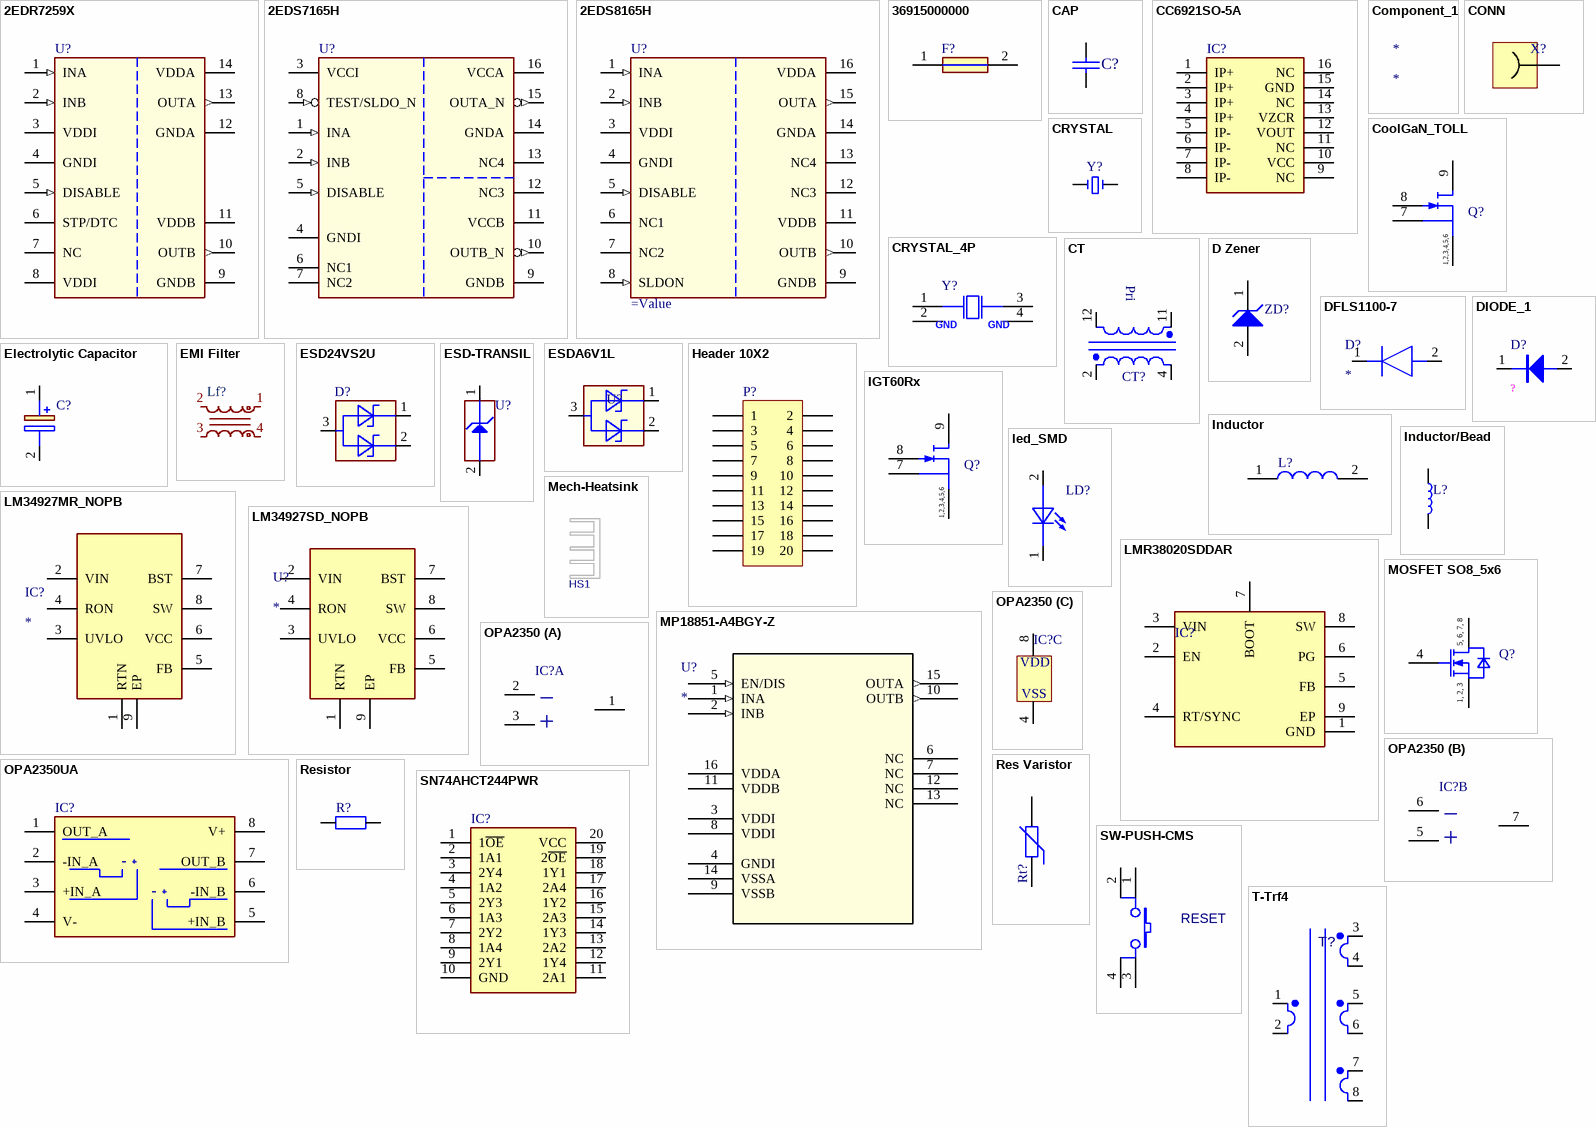
[diagram p0: symbols 2EDR7259X to T-Trf4]
# Altium schematic symbol library MISC82254-2.SchLib: 50 symbols
Pins are listed as number, name and electrical type; pins without a type are passive.


## 2EDR7259X
designator U?
Dual-Channel Isolated Gate Driver
footprint SOIC127P1030X265-16_14N-V (SOIC,1.27mm,pitch;14 pin,7.50mm W X 10.30mm L X 2.65mm H body)
pins: 1 INA (in) "Input signal channel A", 2 INB (in) "Input signal channel B", 3 VDDI (power) "Input-side supply voltage", 4 GNDI (power) "Ground primary-side", 5 DISABLE (in) "Disable input channel A and B", 6 STP/DTC "Shoot-through Protection and Dead-Time Control", 7 NC "No internal connection", 8 VDDI (power) "Input-side supply voltage", 9 GNDB (power) "Ground secondary-side channel B", 10 OUTB (out) "Output secondary-side channel B", 11 VDDB (power) "Supply secondary-side channel B", 12 GNDA (power) "Ground secondary-side channel A", 13 OUTA (out) "Output secondary-side channel A", 14 VDDA (power) "Supply voltage for output channel A"

## 2EDS7165H
designator U?
EiceDRIVER, Two Channel Isolated ISO Driver
footprint SOIC127P1030X265-16N-V (SOIC,1.27mm pitch;16 pin,7.50mm W X 10.30mm L X 2.65mm H body)
pins: 1 INA (in) "Input signal channel A", 2 INB (in) "Input signal channel B", 3 VCCI (power) "Positive supply voltage on input side", 4 GNDI (power) "Ground on input side", 5 DISABLE (in) "Input signal channel A and B", 6 NC1 "Not connected", 7 NC2 "Not connected", 8 TEST/SLDO_N (in) "Switch LDO on, low active or keep it floating / not connected", 9 GNDB (power) "Ground on output side for channel B", 10 OUTB_N (out) "Output driver for channel B", 11 VCCB (power) "Positive supply voltage on output side for channel B", 12 NC3 "Not connected", 13 NC4 "Not connected", 14 GNDA (power) "Ground on output side for channel A", 15 OUTA_N (out) "Output driver for channel A", 16 VCCA (power) "Positive supply voltage on output side for channel A"

## 2EDS8165H
designator U?
Dual-Channel, Functional and Reinforced Isolated MOSFET Gate-Driver
footprint PG-DSO-16 (SOIC,1.27mm pitch;16 pin,7.50mm W X 10.30mm L X 2.65mm H body)
pins: 1 INA (in) "Digital CMOS / TTL logic signal input for channel A with internal pull-down resistor to GNDI", 2 INB (in) "Digital CMOS / TTL logic signal input for channel B with internal pull-down resistor to GNDI", 3 VDDI (power) "Supply voltage (input side) 3.3 V (Internal SLDO available)", 4 GNDI (power) "Ground input side", 5 DISABLE (in) "Digital CMOS / TTL logic input for both channels A and B; logic input high disables both output channels", 6 NC1 "Not connected; keep pin floating", 7 NC2 "Not connected; keep pin floating", 8 SLDON (in) "Default 3.3 V supply selected, if N.C. or connected to VDDI", 9 GNDB (power) "Ground for output channel B", 10 OUTB (out) "Output gate driver for channel B", 11 VDDB (power) "Supply voltage for output channel B", 12 NC3 "Not present; not connected; for channel-to-channel isolation", 13 NC4 "Not connected; for channel-to-channel isolation", 14 GNDA (power) "Ground for output channel A", 15 OUTA (out) "Output gate driver for channel A", 16 VDDA (power) "Supply voltage for output channel A"

## 36915000000
designator F?
Fuse
footprint 36915000000
pins: 1, 2

## CAP
designator C?
footprint 0402C
footprint 0603C
footprint 0805C
footprint 1206C
footprint 1210C (capacitor 1210 reflow soldering)
footprint 2220
footprint CAPE
pins: 1, 2

## CC6921SO-5A
designator IC?
Integrated Circuit
footprint SOIC-16-300mil
pins: 1 IP+, 2 IP+, 3 IP+, 4 IP+, 5 IP-, 6 IP-, 7 IP-, 8 IP-, 9 NC, 10 VCC, 11 NC, 12 VOUT, 13 VZCR, 14 NC, 15 GND, 16 NC

## Component_1
designator *

## CONN
designator X?
footprint CONN_T44008
footprint Con_74650073R
pins: 1

## CoolGaN_TOLL
designator Q?
Field-Effect Transistor (FET), N-Channel, Enhancement, Pin 1-6 Source, Pin 7 kelvin Source, Pin 8 Gate, Pin 9 Drain, 9pins
footprint INF-PG-HSOF-8 (Transistor; 9 pin, 10.375 mm L X 9.90 mm W X 2.40 mm H body)
pins: 1 S1 "Source", 2 S2 "Source", 3 S3 "Source", 4 S4 "Source", 5 S5 "Source", 6 S6 "Source", 7 SK "Kelvin Source", 8 G "Gate", 9 D "DRAIN"

## CRYSTAL
designator Y?
Crystal
footprint XTAL-SMD-NX3215SA-32.768K-STD-MUS-2 (Crystal; 3.2mm W X 1.5mm L X 0.9mm H body)
pins: 1, 2

## CRYSTAL_4P
designator Y?
SMD Crystal Unit for Automotive Application, 12.000MHz; Version Number: V01
footprint XTAL-SMD-NX3225SA
pins: 1, 2 (power) "Ground", 3, 4 (power) "Ground"

## CT
designator CT?
Current transformer
pins: 2, 4, 11, 12

## D Zener
designator ZD?
Zener Diode
simulation model ZENER (Diode)
signal-integrity model D Zener
footprint SOD-323
pins: 1 A, 2 K

## DFLS1100-7
designator D?
Diode
footprint POWERDI123_1
pins: 1 K, 2 A

## DIODE_1
designator D?, comment ?
footprint SOD-323
footprint POWERDI123_1
footprint SMA
footprint SMA_L4.3-W2.6-LS5.2-RD
pins: 1 K, 2 A

## Electrolytic Capacitor
designator C?
Capacitor Polarised
footprint CAPPRD1000W190D3575H3200
pins: 1 +, 2 -

## EMI Filter
designator Lf?
pins: 1, 2, 3, 4

## ESD24VS2U
designator D?
Silicon TVS Diode, VRWM 24V
footprint SOT95P240X110-3N-1-V
pins: 1 CATHODE1 "Cathode", 2 CATHODE2 "Cathode", 3 ANODE "Anode"

## ESD-TRANSIL
designator U?
ESD protection 6V1
footprint ESD_ST0201
pins: 1 IO1, 2 GND

## ESDA6V1L
designator U?
No Description Available
footprint SOT_DA6V1L_STM
pins: 1 CATHODE1 "Cathode", 2 CATHODE2 "Cathode", 3 ANODE "Anode"

## Header 10X2
designator P?
Header, 10-Pin, Dual row
footprint HDR2X10 (Connector; Header; 10x2 Position)
pins: 1, 2, 3, 4, 5, 6, 7, 8, 9, 10, 11, 12, 13, 14, 15, 16, 17, 18, 19, 20

## IGT60Rx
designator Q?
Field-Effect Transistor (FET), N-Channel, Enhancement, Pin 1-6 Source, Pin 7 kelvin Source, Pin 8 Gate, Pin 9 Drain, 9pins
footprint INF-PG-HSOF-8 (Transistor; 9 pin, 10.375 mm L X 9.90 mm W X 2.40 mm H body)
pins: 1 S1 "Source", 2 S2 "Source", 3 S3 "Source", 4 S4 "Source", 5 S5 "Source", 6 S6 "Source", 7 SK "Kelvin Source", 8 G "Gate", 9 D "DRAIN"

## Inductor
designator L?
Inductor
pins: 1, 2

## Inductor/Bead
designator L?
footprint 0603R
pins: 1, 2
2 alternate drawings of the same symbol

## led_SMD
designator LD?
Version Number: V01
footprint LED0603-RD
pins: 1 Cathode, 2 Anode

## LM34927MR_NOPB
designator IC?
Integrated Circuit
footprint SOIC127P600X170-9N
pins: 1 RTN, 2 VIN, 3 UVLO, 4 RON, 5 FB, 6 VCC, 7 BST, 8 SW, 9 EP

## LM34927SD_NOPB
designator U?
Integrated Circuit
footprint WSON8
pins: 1 RTN, 2 VIN, 3 UVLO, 4 RON, 5 FB, 6 VCC, 7 BST, 8 SW, 9 EP

## LMR38020SDDAR
designator IC?
Integrated Circuit
footprint SO-8-PowerPad
pins: 1 GND, 2 EN, 3 VIN, 4 RT/SYNC, 5 FB, 6 PG, 7 BOOT, 8 SW, 9 EP

## Mech-Heatsink
designator HS1
Heatsink kit with Heatsink, Silpad and Clip
footprint Heatsink 15x15
footprint Heatsink 16x36x12(h) (4mm elevated)
footprint Heatsink 39x27.5mm (Manufactured from CTS BDN18-6CB/A01)
footprint Heatsink 46x28.5mm (Manufactured from CTS BDN18-6CB/A01)
footprint Heatsink 55x28.5 (1mm copper sheet)
footprint Heatsink C1613-001-04

## MOSFET SO8_5x6
designator Q?
MOSFET SO8 5x6
footprint IFX-PG-TDSON-8-36-V (PG-TDSON-8-36, SMD, 1.27 mm pitch, 8 pin, 5.90 mm L X 5.15 mm W X 1.00 mm H body)
pins: 1 SOURCE, 2 SOURCE, 3 SOURCE, 4 GATE, 5 DRAIN, 6 DRAIN, 7 DRAIN, 8 DRAIN

## MP18851-A4BGY-Z
designator U?
No Description Available
footprint SOIC-16WB_MP18851_MNP
pins: 1 INA (in), 2 INB (in), 3 VDDI (power), 4 GNDI (power), 5 EN/DIS (in), 6 NC, 7 NC, 8 VDDI (power), 9 VSSB (power), 10 OUTB (out), 11 VDDB (power), 12 NC, 13 NC, 14 VSSA (power), 15 OUTA (out), 16 VDDA (power)

## OPA2350
designator IC?
Dual op amp
footprint SOIC127P600X175-8N
part A pins: 1, 2, 3
part B pins: 5, 6, 7
part C pins: 4, 8

## OPA2350UA
designator IC?
Integrated Circuit
footprint SOIC127P600X175-8N
pins: 1 OUT_A, 2 -IN_A, 3 +IN_A, 4 V-, 5 +IN_B, 6 -IN_B, 7 OUT_B, 8 V+

## Res Varistor
designator Rt?
Thermistor
footprint RES-TH_Vol
footprint RV1-7.5MM
footprint R0603T
footprint 0603R
pins: 1, 2

## Resistor
designator R?
Resistor
signal-integrity model Res
simulation model RESISTOR
footprint 0402R
footprint 0603R
footprint 0805R
footprint 1206R
footprint 1210R
footprint 2220
pins: 1, 2

## SN74AHCT244PWR
designator IC?
Integrated Circuit
footprint TSSOP-20_L6.5-W4.4-P0.65-LS6.4-BL
pins: 1 1~{OE}, 2 1A1, 3 2Y4, 4 1A2, 5 2Y3, 6 1A3, 7 2Y2, 8 1A4, 9 2Y1, 10 GND, 11 2A1, 12 1Y4, 13 2A2, 14 1Y3, 15 2A3, 16 1Y2, 17 2A4, 18 1Y1, 19 2~{OE}, 20 VCC

## SW-PUSH-CMS
designator RESET
Non-Open Push-Button 0.1A 24V BLACK
footprint PTS647SM38SMTR2LFS
pins: 1, 2, 3, 4

## T-Trf4
designator T?
MAG-1238 13V to 12V
footprint Trans_isoBuck_MOS - EE25/20
pins: 1, 2, 3, 4, 5, 6, 7, 8

## T-Trf6
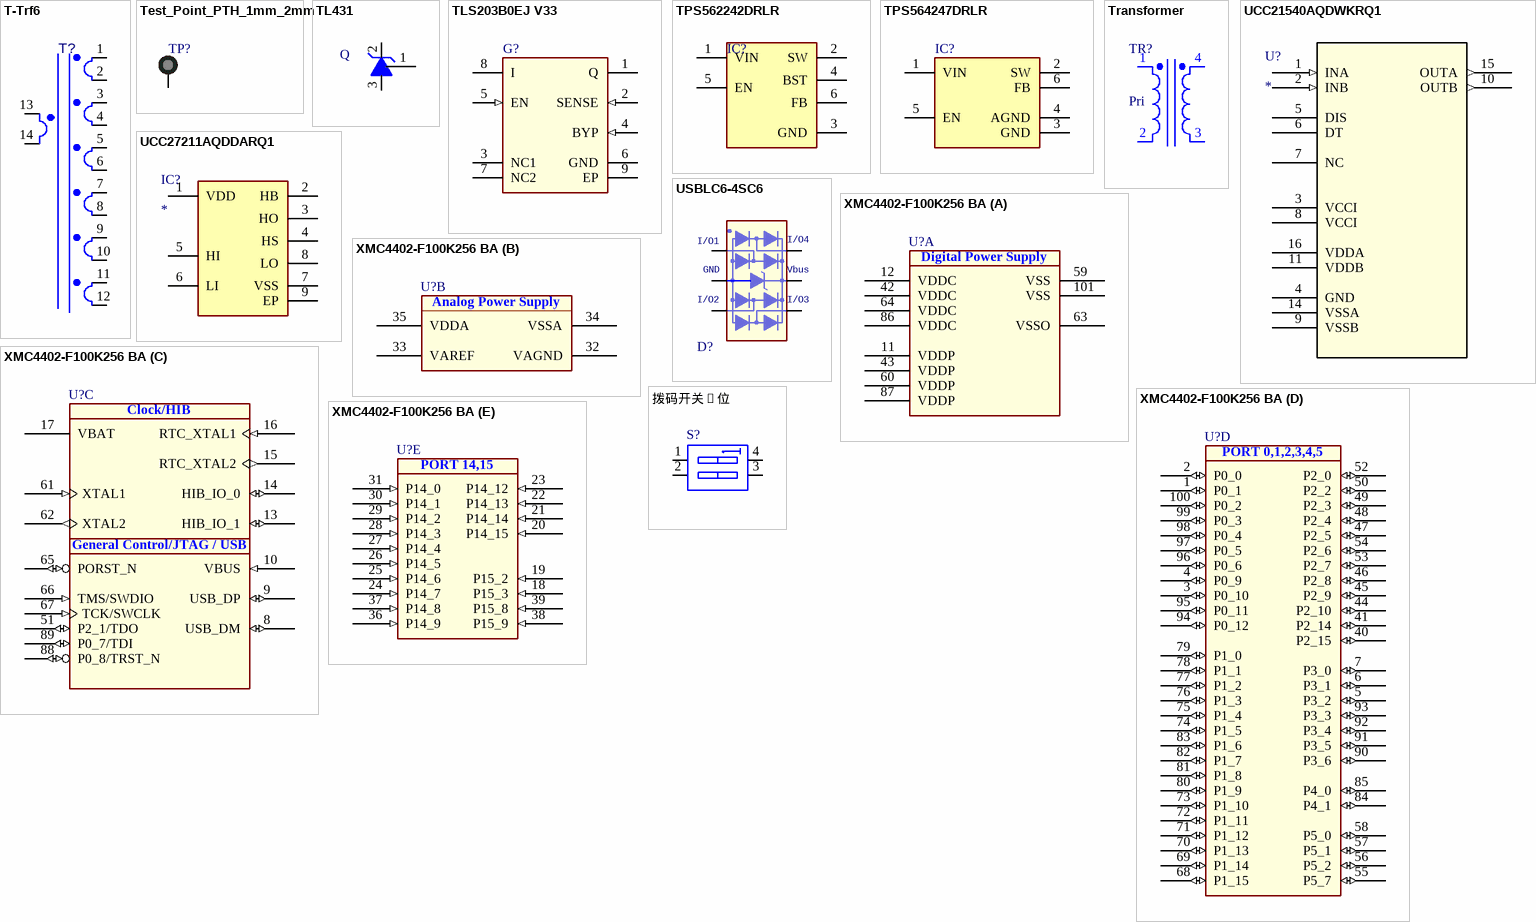
[diagram p1: symbols T-Trf6 to 拨码开关2位]
## T-Trf6
designator T?
MAG-1238 13V to 12V
footprint ER9.5/5 (8 pin SM ER9.5/5)
footprint ER9.5/5 - Buried (8 pin SM ER9.5/5 - Fits in PCB cutout with bottom side pads)
pins: 1, 2, 3, 4, 5, 6, 7, 8, 9, 10, 11, 12, 13 14, 14

## Test_Point_PTH_1mm_2mm
designator TP?
Test Point trought hole 1mm/2mm
footprint TP_PTH_1MM_2MM
pins: 1

## TL431
designator Q
Three-terminal voltage regulator, 1.25V
footprint TL431 (SOT23, 3-Leads, Body 2.92x2.37mm, Pitch 0.95mm, IPC Medium Density)
pins: 1 REFERENCE, 2 CATHODE, 3 ANODE

## TLS203B0EJ V33
designator G?
Low Dropout, Low Noise, Linear Voltage Post Regulator, 3.3V, 500 mA
footprint SOIC127P600X170-9N-3-V1 (SOIC,1.27mm pitch;8 pin,3.90mm W X 4.90mm L X 1.70mm H body (w/thermal tab))
pins: 1 Q (power) "Output", 2 SENSE (in) "Output Sense", 3 NC1 "Not connected", 4 BYP (in) "Bypass", 5 EN (in) "Enable", 6 GND (power) "Ground", 7 NC2 "Not connected", 8 I (power) "Input", 9 EP (power) "Exposed Pad"

## TPS562242DRLR
designator IC?
Integrated Circuit
footprint SOTFL50P160X60-6N
pins: 1 VIN, 2 SW, 3 GND, 4 BST, 5 EN, 6 FB

## TPS564247DRLR
designator IC?
Integrated Circuit
footprint SOTFL50P160X60-6N
pins: 1 VIN, 2 SW, 3 GND, 4 AGND, 5 EN, 6 FB

## Transformer
designator TR?
1:5
pins: 1, 2, 3, 4

## UCC21540AQDWKRQ1
designator U?
No Description Available
footprint SOIC_WKRQ1_TEX
pins: 1 INA (in), 2 INB (in), 3 VCCI (power), 4 GND (power), 5 DIS, 6 DT, 7 NC, 8 VCCI (power), 9 VSSB (power), 10 OUTB (out), 11 VDDB (power), 14 VSSA (power), 15 OUTA (out), 16 VDDA (power)

## UCC27211AQDDARQ1
designator IC?
Integrated Circuit
footprint SOIC8 Powerpad
pins: 1 VDD, 2 HB, 3 HO, 4 HS, 5 HI, 6 LI, 7 VSS, 8 LO, 9 EP

## USBLC6-4SC6
designator D?
footprint ST_SOT23-6L
pins: 1 I/O1, 2 GND, 3 I/O2, 4 I/O3, 5 Vbus, 6 I/O4

## XMC4402-F100K256 BA
designator U?
XMC4000 Family Microcontroller for Industrial Applications, ARM® Cortex™-M4, 32-bit processor coreFlash 1536 Kbytes,SRAM 276 Kbytes (Temperature Range -40°C to 85°C)
footprint QFP50P1600X1600X160-101N-V (QFP,0.50mm pitch,square;100 pin,14.00mm L X 14.00mm W X 1.60mm H body (w/thermal tab))
part A pins: 11 VDDP (power), 12 VDDC (power), 42 VDDC (power), 43 VDDP (power), 59 VSS (power), 60 VDDP (power), 63 VSSO (power), 64 VDDC (power), 86 VDDC (power), 87 VDDP (power), 101 VSS (power) "Exposed Pad"
part B pins: 32 VAGND (power), 33 VAREF (power), 34 VSSA (power), 35 VDDA (power)
part C pins: 8 USB_DM (io), 9 USB_DP (io), 10 VBUS (in), 13 HIB_IO_1 (io), 14 HIB_IO_0 (io), 15 RTC_XTAL2 (out), 16 RTC_XTAL1 (in), 17 VBAT (power), 51 P2_1/TDO (io), 61 XTAL1 (in), 62 XTAL2 (out), 65 PORST_N (io), 66 TMS/SWDIO (in), 67 TCK/SWCLK (in), 88 P0_8/TRST_N (io), 89 P0_7/TDI (io)
part D pins: 1 P0_1 (io), 2 P0_0 (io), 3 P0_10 (io), 4 P0_9 (io), 5 P3_2 (io), 6 P3_1 (io), 7 P3_0 (io), 40 P2_15 (io), 41 P2_14 (io), 44 P2_10 (io), 45 P2_9 (io), 46 P2_8 (io), 47 P2_5 (io), 48 P2_4 (io), 49 P2_3 (io), 50 P2_2 (io), 52 P2_0 (io), 53 P2_7 (io), 54 P2_6 (io), 55 P5_7 (io), 56 P5_2 (io), 57 P5_1 (io), 58 P5_0 (io), 68 P1_15 (io), 69 P1_14 (io), 70 P1_13 (io), 71 P1_12 (io), 72 P1_11 (io), 73 P1_10 (io), 74 P1_5 (io), 75 P1_4 (io), 76 P1_3 (io), 77 P1_2 (io), 78 P1_1 (io), 79 P1_0 (io), 80 P1_9 (io), 81 P1_8 (io), 82 P1_7 (io), 83 P1_6 (io), 84 P4_1 (io), 85 P4_0 (io), 90 P3_6 (io), 91 P3_5 (io), 92 P3_4 (io), 93 P3_3 (io), 94 P0_12 (io), 95 P0_11 (io), 96 P0_6 (io), 97 P0_5 (io), 98 P0_4 (io), 99 P0_3 (io), 100 P0_2 (io)
part E pins: 18 P15_3 (in), 19 P15_2 (in), 20 P14_15 (in), 21 P14_14 (in), 22 P14_13 (in), 23 P14_12 (in), 24 P14_7 (in), 25 P14_6 (in), 26 P14_5 (in), 27 P14_4 (in), 28 P14_3 (in), 29 P14_2 (in), 30 P14_1 (in), 31 P14_0 (in), 36 P14_9 (in), 37 P14_8 (in), 38 P15_9 (in), 39 P15_8 (in)

## 拨码开关2位
designator S?
拨码开关EM-02
footprint SW-SMD_4P_DSHP02TSGET
pins: 1 A1, 2 A2, 3 B2, 4 B1